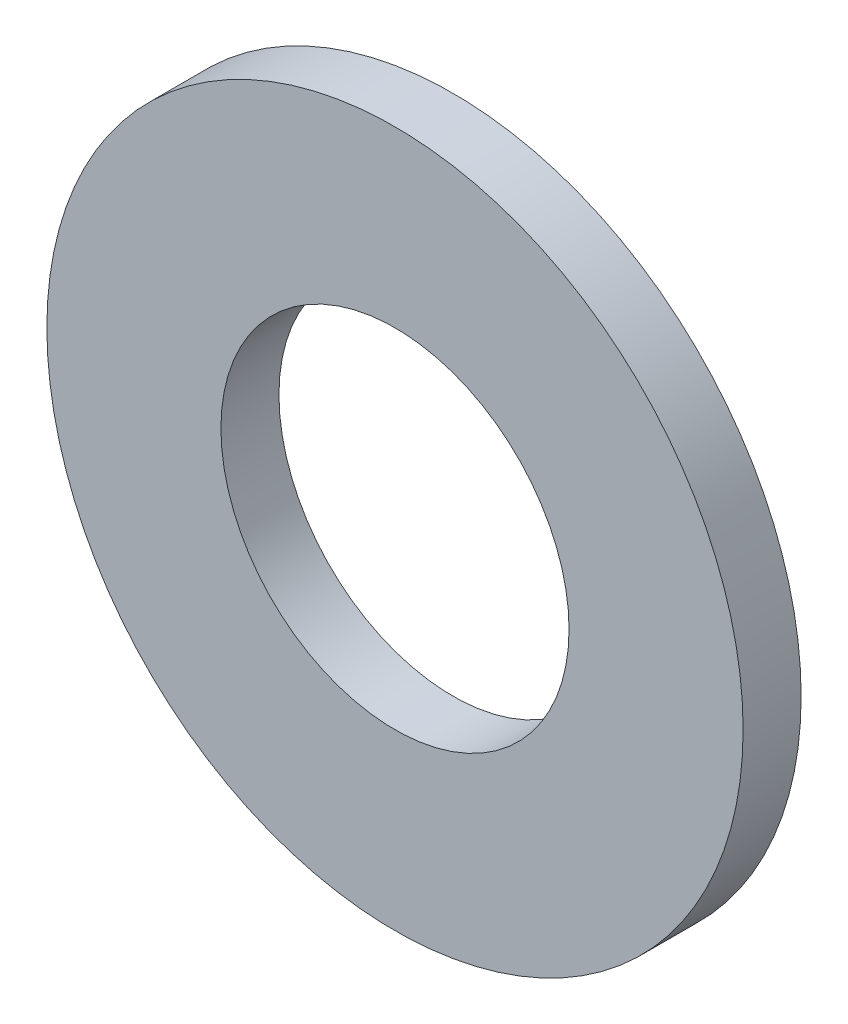
SolidWorks part; units mm, degrees
material "Q235-A"
ref_plane "Front Plane" through (0, 0, 0) normal (0, 0, 1) x (1, 0, 0)
ref_plane "Top Plane" through (0, 0, 0) normal (0, 1, 0) x (1, 0, 0)
ref_plane "Right Plane" through (0, 0, 0) normal (1, 0, 0) x (0, 0, -1)
sketch "Sketch1" plane through (0, 0, 0) normal (0, 0, 1) x (1, 0, 0)
  circle A0 centre (0, 0) radius 24
  circle A1 centre (0, 0) radius 12
extrude "Boss-Extrude1" add sketch "Sketch1" along normal blind 4
